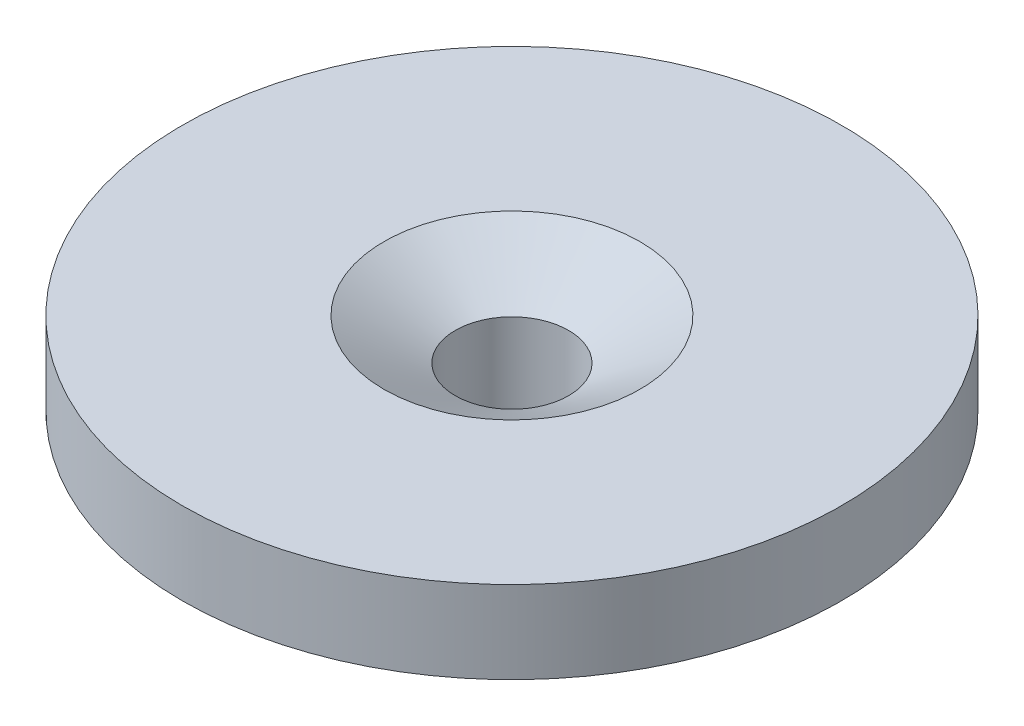
SolidWorks part; units mm, degrees
ref_plane "Front Plane" through (0, 0, 0) normal (0, 0, 1) x (1, 0, 0)
ref_plane "Top Plane" through (0, 0, 0) normal (0, 1, 0) x (1, 0, 0)
ref_plane "Right Plane" through (0, 0, 0) normal (1, 0, 0) x (0, 0, -1)
other "Configuration Table"
sketch "Sketch1" plane through (0, 0, 0) normal (0, 0, 1) x (1, 0, 0)
  line L0 (0, 9.9089) -> (0, -11.3108) construction
  line L1 (-2.75, -2.2262) -> (-9, -2.2262)
  line L2 (-9, -2.2262) -> (-9, 1.7738)
  line L3 (-9, 1.7738) -> (-14, 1.7738)
  line L4 (-14, 1.7738) -> (-14, -0.2262)
  line L5 (-14, -0.2262) -> (-16, -0.2262)
  line L6 (-16, -0.2262) -> (-16, 3.7738)
  line L7 (-16, 3.7738) -> (-6.2141, 3.7738)
  line L8 (-2.75, -2.2262) -> (-2.75, 1.7738)
  line L10 (-2.75, 1.7738) -> (-6.2141, 3.7738)
  dimension "D1" = 6
  dimension "D2" = 4
  dimension "D3" = 14
  dimension "D4" = 16
  dimension "D5" = 9
  dimension "D6" = 4
  dimension "D7" = 4
  dimension "D8" = 60
revolve "Revolve1" add sketch "Sketch1" angle 360 about L0
